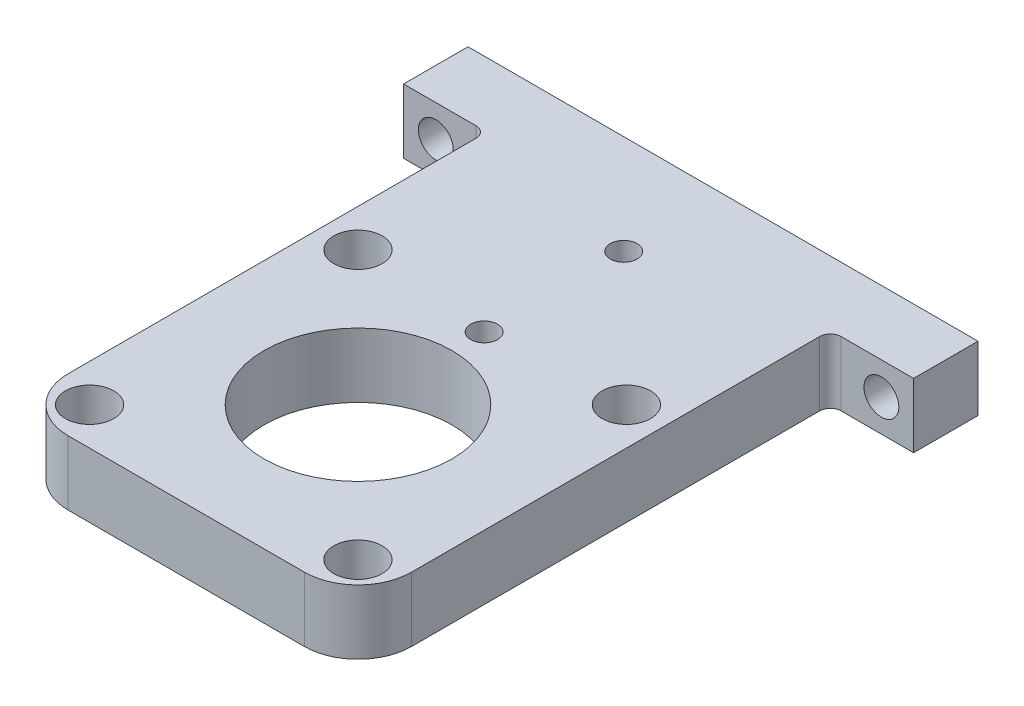
SolidWorks part; units mm, degrees
material "45钢"
ref_plane "前视基准面" through (0, 0, 0) normal (0, 0, 1) x (1, 0, 0)
ref_plane "上视基准面" through (0, 0, 0) normal (0, 1, 0) x (1, 0, 0)
ref_plane "右视基准面" through (0, 0, 0) normal (1, 0, 0) x (0, 0, -1)
sketch "草图1" plane through (0, 0, 0) normal (0, 1, 0) x (1, 0, 0)
  line L0 (0, 0) -> (95, 0)
  line L1 (95, 0) -> (95, -100)
  line L4 (95, -100) -> (0, -100)
  line L5 (0, -100) -> (0, 0)
  dimension "D1" = 95
  dimension "D2" = 100
extrude "凸台-拉伸1" add sketch "草图1" along normal blind 12
hole_wizard "Ø16.0 (16) 直径孔1" positions "草图6" profile "草图5" hole size "Ø16.0" standard "GB"
sketch "草图6" plane through (0, 15, 0) normal (0, 1, 0) x (1, 0, 0)
  line L0 (70, 0) -> (0, 0) construction
  line L2 (35, -31) -> (35, -52) construction
  line L3 (0, -52) -> (70, -52) construction
  point P0 (35, -31)
  dimension "D1" = 31
sketch "草图5" plane through (35, 15, 31) normal (1, 0, 0) x (0, 0, 1)
  line L0 (0, 0) -> (0, 15)
  line L1 (0, 15) -> (8.1, 15)
  line L2 (8.1, 15) -> (8.1, 0)
  line L5 (8.1, 0) -> (0, 0)
  line L11 (0, -6.35) -> (0, 107.95) construction
  dimension "通孔孔直径" = 16.2
  dimension "通孔孔深度" = 15
sketch "草图8" [suppressed] plane through (0, 0, 0) normal (0, -1, 0) x (1, 0, 0)
  line L1 (-59.908, 80.8452) -> (106.3415, 80.8452)
  line L2 (-59.908, 80.8452) -> (-59.908, 14)
  line L3 (-59.908, 14) -> (106.3415, 14)
  line L4 (106.3415, 80.8452) -> (106.3415, 14)
  line L5 (-59.908, 80.8452) -> (106.3415, 14) construction
  line L6 (-59.908, 14) -> (106.3415, 80.8452) construction
  circle A0 centre (35, 31) radius 8.1 construction
  point P0 (23.2167, 47.4226)
  dimension "D1" = 17
extrude "切除-拉伸3" [suppressed] cut sketch "草图8" against normal offset from surface (6 mm away) 9
ref_plane "基准面1" through (47.5, 0, 0) normal (-1, 0, 0) x (0, 0, 1)
sketch "草图9" plane through (0, 12, 0) normal (0, 1, 0) x (1, 0, 0)
  line L0 (95, 0) -> (0, 0) construction
  line L1 (0, -100) -> (15.5, -100)
  line L2 (0, -100) -> (0, -12)
  line L3 (0, -12) -> (15.5, -12)
  line L4 (15.5, -100) -> (15.5, -12)
  line L5 (95, -100) -> (79.5, -100)
  line L6 (95, -100) -> (95, -12)
  line L7 (95, -12) -> (79.5, -12)
  line L8 (79.5, -100) -> (79.5, -12)
  dimension "D1" = 64
  dimension "D2" = 12
extrude "切除-拉伸4" cut sketch "草图9" against normal through all
hole_wizard "Ø6.5 (6.5) 直径孔1" positions "草图10" profile "草图11" hole size "Ø6.5" standard "GB" end condition through all
sketch "草图10" plane through (0, 0, 12) normal (0, 0, 1) x (1, 0, 0)
  line L0 (0, 6) -> (6, 6) construction
  line L1 (0, 0) -> (0, 12) construction
  line L2 (6, 6) -> (89, 6) construction
  line L3 (89, 6) -> (95, 6) construction
  line L4 (95, 0) -> (95, 12) construction
  point P0 (6, 6)
  point P2 (89, 6)
  dimension "D1" = 6
sketch "草图11" plane through (6, 6, 12) normal (1, 0, 0) x (0, -1, 0)
  line L0 (0, 0) -> (0, 12)
  line L1 (0, 12) -> (3.25, 12)
  line L2 (3.25, 12) -> (3.25, 0)
  line L5 (3.25, 0) -> (0, 0)
  line L11 (0, -6.35) -> (0, 107.95) construction
  dimension "通孔孔直径" = 6.5
  dimension "通孔孔深度" = 12
sketch "草图12" plane through (0, 12, 0) normal (0, 1, 0) x (1, 0, 0)
  line L0 (47.5, 0) -> (47.5, -68) construction
  line L1 (95, 0) -> (0, 0) construction
  circle A0 centre (47.5, -68) radius 17.5
  dimension "D2" = 35
  dimension "D1" = 68
extrude "切除-拉伸5" cut sketch "草图12" against normal through all
fillet "圆角1" radius 10 2 edges at (15.5, 6, 100) (79.5, 6, 100)
hole_wizard "Ø5.0 (5) 直径孔1" positions "草图13" profile "草图14" hole size "Ø5.0" standard "GB"
sketch "草图13" plane through (0, 0, 0) normal (0, 0, -1) x (-1, 0, 0)
  line L0 (-47.5, 12) -> (-47.5, -2.6375) construction
  line L1 (-95, 12) -> (0, 12) construction
  line L4 (-67.5, 6) -> (-27.5, 6) construction
  line L5 (-27.5, 6) -> (0, 6) construction
  line L6 (0, 12) -> (0, 0) construction
  point P0 (-67.5, 6)
  point P2 (-27.5, 6)
  dimension "D1" = 40
sketch "草图14" plane through (67.5, 6, 0) normal (1, 0, 0) x (0, 1, 0)
  line L0 (0, 0) -> (0, 11.5022)
  line L1 (0, 11.5022) -> (2.5, 10)
  line L2 (2.5, 10) -> (2.5, 0)
  line L5 (2.5, 0) -> (0, 0)
  line L10 (0, 11.5022) -> (-2.5, 10) construction
  line L11 (0, -6.35) -> (0, 107.95) construction
  dimension "孔直径" = 5
  dimension "孔深度" = 10
  dimension "导头角度" = 118
fillet "圆角2" radius 2 2 edges at (15.5, 6, 12) (79.5, 6, 12)
hole_wizard "大小mm 暗销孔1" positions "草图17" profile "草图19" hole size "Ø5.0" standard "GB" end condition through all
sketch "草图17" plane through (0, 0, 0) normal (0, -1, 0) x (-1, 0, 0)
  point P0 (-72.5, -43)
  point P3 (-72.5, -93)
  point P6 (-22.5, -93)
  point P9 (-22.5, -43)
sketch "草图19" plane through (72.5, 0, 43) normal (1, 0, 0) x (0, 0, -1)
  line L0 (0, 0) -> (0, 12)
  line L1 (0, 12) -> (4.5, 12)
  line L2 (4.5, 12) -> (4.5, 0)
  line L5 (4.5, 0) -> (0, 0)
  line L11 (0, -6.35) -> (0, 107.95) construction
  dimension "通孔孔直径" = 9
  dimension "通孔孔深度" = 12
hole_wizard "M6 螺纹孔1" positions "草图20" profile "草图21" tap size "M6" standard "GB" end condition through all
sketch "草图20" plane through (0, 0, 0) normal (0, -1, 0) x (-1, 0, 0)
  line L0 (-47.5, -68) -> (-47.5, -27.13) construction
  line L1 (-25.5, -100) -> (-69.5, -100) construction
  point P6 (-47.5, -44.5)
  dimension "D1" = 55.5
sketch "草图21" plane through (47.5, 0, 44.5) normal (1, 0, 0) x (0, 0, -1)
  line L0 (0, 0) -> (0, 12)
  line L1 (0, 12) -> (2.5, 12)
  line L2 (2.5, 12) -> (2.5, 0)
  line L5 (2.5, 0) -> (0, 0)
  line L11 (0, -6.35) -> (0, 107.95) construction
  dimension "通孔螺纹孔钻头直径" = 5
  dimension "通孔螺纹孔钻头深度" = 12
cosmetic thread "孔螺蚊线1" parameters "D2"=6
hole_wizard "M6 螺纹孔2" positions "草图23" profile "草图24" tap size "M6" standard "GB" end condition through all
sketch "草图23" plane through (0, 0, 0) normal (0, -1, 0) x (-1, 0, 0)
  line L0 (-47.5, -20) -> (-47.5, -17) construction
  point P7 (-47.5, -18.5)
sketch "草图24" plane through (47.5, 0, 18.5) normal (1, 0, 0) x (0, 0, -1)
  line L0 (0, 0) -> (0, 12)
  line L1 (0, 12) -> (2.5, 12)
  line L2 (2.5, 12) -> (2.5, 0)
  line L5 (2.5, 0) -> (0, 0)
  line L11 (0, -6.35) -> (0, 107.95) construction
  dimension "通孔螺纹孔钻头直径" = 5
  dimension "通孔螺纹孔钻头深度" = 12
cosmetic thread "孔螺蚊线2" parameters "D2"=6
